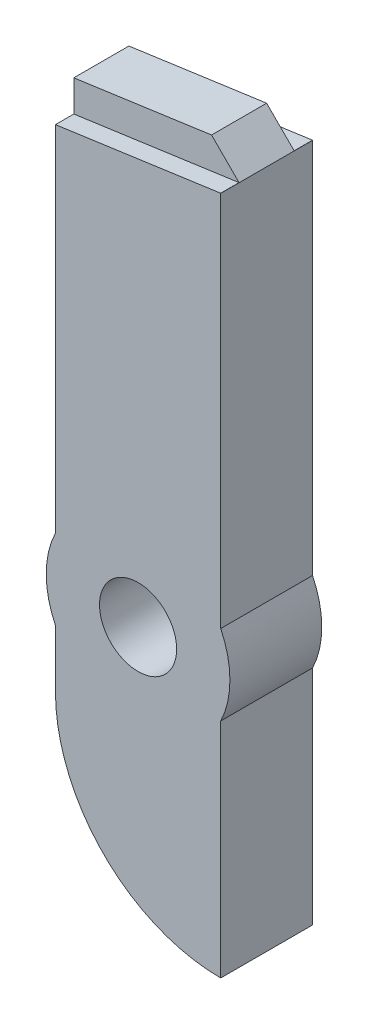
from build123d import *

# Parameters (mm, degrees)
SKETCH_1_R               = 21
EXTRUDE_1_DEPTH          = 25
CUT_EXTRUDE_1_DEPTH      = 396.281407624
CUT_EXTRUDE_1_DEPTH_BACK = 396.281407624
SKETCH_2_W               = 10
SKETCH_2_H               = 16.9


with BuildPart() as part:
    # 草图1 → 凸台-拉伸1 (new, symmetric)
    with BuildSketch(Plane.XY):
        with BuildLine():
            Line((0, 0), (0, 121.205505282))
            ThreePointArc((0, 121.205505282), (5, 143), (0, 164.794494718))
            Line((0, 164.794494718), (0, 370))
            Line((0, 370), (-15, 385))
            Line((-15, 385), (-90, 374.459437397))
            Line((-90, 374.459437397), (-90, 164.794494718))
            ThreePointArc((-90, 164.794494718), (-95, 143), (-90, 121.205505282))
            Line((-90, 121.205505282), (-90, 90))
            ThreePointArc((-90, 90), (-63.639610307, 26.360389693), (0, 0))
        make_face()
        with Locations((-45, 143)):
            Circle(SKETCH_1_R, mode=Mode.SUBTRACT)
    extrude(amount=EXTRUDE_1_DEPTH, both=True)

    # 草图2 → 切除-拉伸1 (cut, two sides: drawn at the far end of the back side and taken through both)
    with BuildSketch(Plane(origin=(-36.649271725, -5.150719239, 0), x_dir=(0, 0, -1), z_dir=(0.9902680687415697, 0.1391731009600695, 0)).offset(-CUT_EXTRUDE_1_DEPTH_BACK)):
        with Locations((-20, 374.89080298)):
            Rectangle(SKETCH_2_W, SKETCH_2_H)
        with Locations((20, 374.89080298)):
            Rectangle(SKETCH_2_W, SKETCH_2_H)
    extrude(amount=CUT_EXTRUDE_1_DEPTH + CUT_EXTRUDE_1_DEPTH_BACK, mode=Mode.SUBTRACT)


solid = part.part
